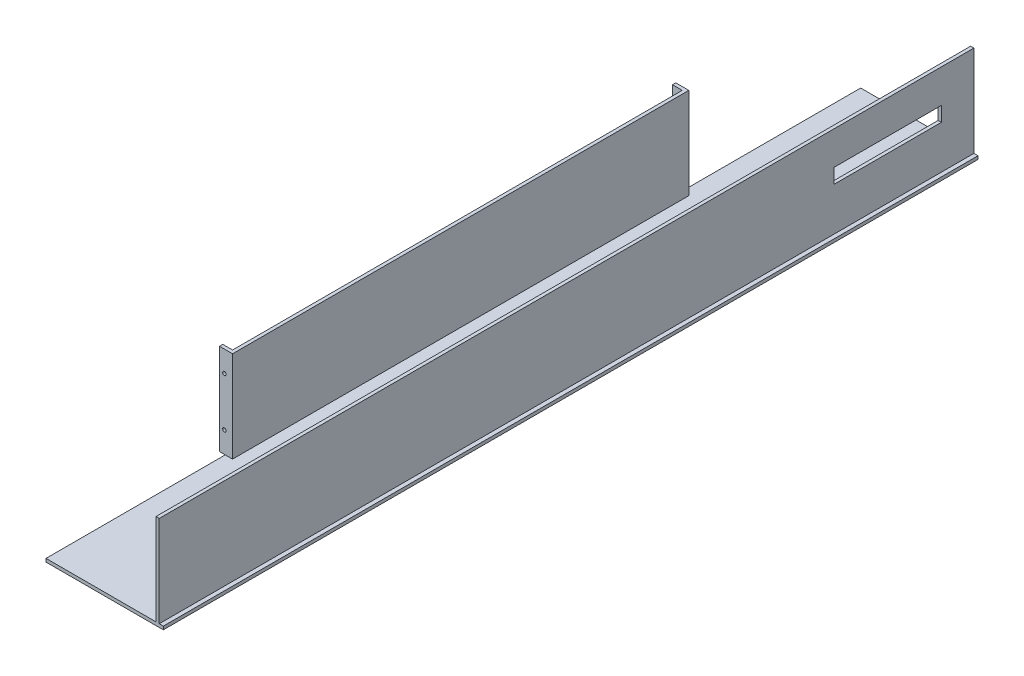
SolidWorks part; units mm, degrees
ref_plane "Front Plane" through (0, 0, 0) normal (0, 0, 1) x (1, 0, 0)
ref_plane "Top Plane" through (0, 0, 0) normal (0, 1, 0) x (1, 0, 0)
ref_plane "Right Plane" through (0, 0, 0) normal (1, 0, 0) x (0, 0, -1)
other "Configuration Table"
sketch "Sketch1" plane through (0, 0, 0) normal (0, 0, 1) x (1, 0, 0)
  line L0 (0, 0) -> (0, 470.1987) construction
  line L1 (360, 0) -> (-360, 0)
  line L2 (-360, 0) -> (-360, 20)
  line L3 (-360, 20) -> (-335, 20)
  line L4 (-335, 20) -> (-335, 580)
  line L5 (-335, 580) -> (-315, 580)
  line L6 (-315, 580) -> (-315, 20)
  line L7 (-315, 20) -> (315, 20)
  line L8 (315, 580) -> (315, 20)
  line L9 (335, 580) -> (315, 580)
  line L10 (335, 20) -> (335, 580)
  line L11 (360, 20) -> (335, 20)
  line L12 (360, 0) -> (360, 20)
  point P11 (0, 20)
  dimension "D1" = 720
  dimension "D2" = 560
  dimension "D3" = 20
  dimension "D4" = 20
  dimension "D5" = 315
extrude "Boss-Extrude1" add sketch "Sketch1" along normal blind 5000
sketch "Sketch2" plane through (335, 0, 0) normal (1, 0, 0) x (0, 0, -1)
  line L1 (-5000, 20) -> (0, 20) construction
  line L2 (-860, 375) -> (-200, 375)
  line L3 (-860, 375) -> (-860, 285)
  line L4 (-860, 285) -> (-200, 285)
  line L5 (-200, 375) -> (-200, 285)
  line L6 (-860, 375) -> (-200, 285) construction
  line L7 (-860, 285) -> (-200, 375) construction
  line L8 (0, 20) -> (0, 580) construction
  point P0 (-530, 330)
  dimension "D1" = 310
  dimension "D2" = 90
  dimension "D3" = 660
  dimension "D4" = 200
extrude "Cut-Extrude1" cut sketch "Sketch2" against normal up to next
sketch "Sketch3" plane through (-335, 0, 0) normal (-1, 0, 0) x (0, 0, 1)
  line L0 (5000, 20) -> (0, 20) construction
  line L1 (5000, 580) -> (3900, 580)
  line L2 (5000, 580) -> (5000, 20)
  line L3 (5000, 20) -> (3900, 20)
  line L4 (3900, 580) -> (3900, 20)
  line L5 (0, 580) -> (1100, 580)
  line L6 (0, 580) -> (0, 20)
  line L7 (0, 20) -> (1100, 20)
  line L8 (1100, 580) -> (1100, 20)
  dimension "D1" = 1100
  dimension "D2" = 1100
extrude "Cut-Extrude2" cut sketch "Sketch3" against normal blind 20
sketch "Sketch4" plane through (-335, 0, 0) normal (-1, 0, 0) x (0, 0, 1)
  line L0 (3900, 20) -> (1100, 20) construction
  line L1 (1100, 580) -> (1120, 580)
  line L2 (1100, 580) -> (1100, 20)
  line L3 (1100, 20) -> (1120, 20)
  line L4 (1120, 580) -> (1120, 20)
  line L6 (3900, 580) -> (3880, 580)
  line L7 (3900, 580) -> (3900, 20)
  line L8 (3900, 20) -> (3880, 20)
  line L9 (3880, 580) -> (3880, 20)
  dimension "D1" = 20
  dimension "D2" = 20
extrude "Boss-Extrude2" add sketch "Sketch4" along normal blind 60
sketch "Sketch5" plane through (0, 0, 3900) normal (0, 0, 1) x (1, 0, 0)
  line L0 (-395, 20) -> (-395, 580) construction
  line L1 (-315, 580) -> (-395, 580) construction
  circle A0 centre (-365, 450) radius 11
  circle A1 centre (-365, 150) radius 11
  dimension "D1" = 22
  dimension "D2" = 22
  dimension "D3" = 30
  dimension "D4" = 30
  dimension "D5" = 130
  dimension "D6" = 300
extrude "Cut-Extrude3" cut sketch "Sketch5" against normal through all
